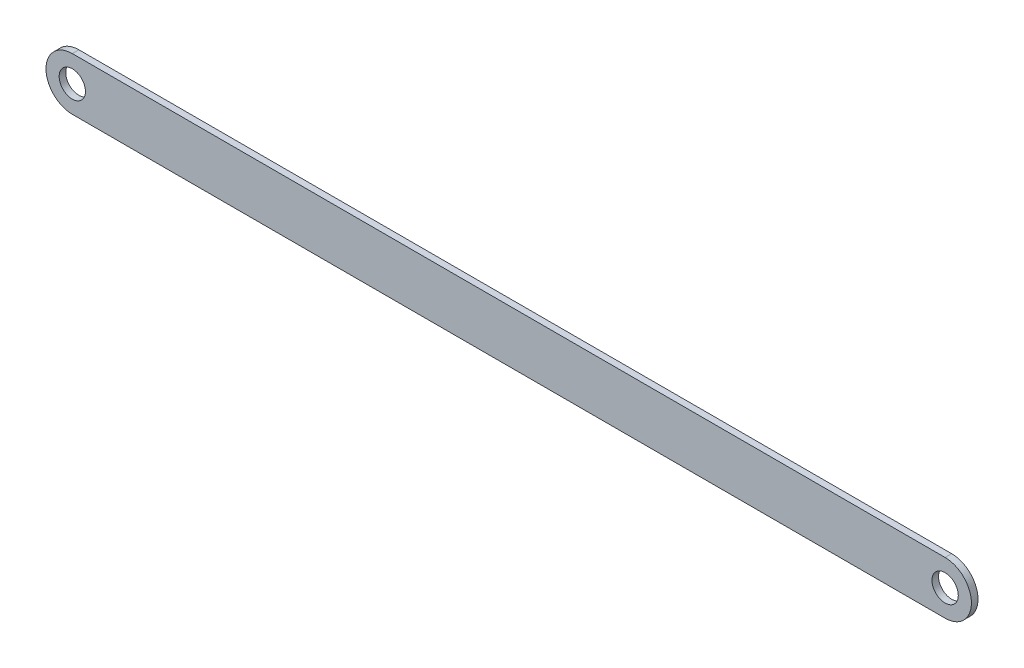
SolidWorks part; units mm, degrees
ref_plane "Front Plane" through (0, 0, 0) normal (0, 0, 1) x (1, 0, 0)
ref_plane "Top Plane" through (0, 0, 0) normal (0, 1, 0) x (1, 0, 0)
ref_plane "Right Plane" through (0, 0, 0) normal (1, 0, 0) x (0, 0, -1)
sketch "Sketch1" plane through (0, 0, 0) normal (0, 0, 1) x (1, 0, 0)
  line L0 (-165.885, 0) -> (165.885, 0) construction
  line L1 (-165.885, 10) -> (165.885, 10)
  line L2 (-165.885, -10) -> (165.885, -10)
  arc A0 (-165.885, 10) -> (-165.885, -10) centre (-165.885, 0) ccw
  arc A1 (165.885, -10) -> (165.885, 10) centre (165.885, 0) ccw
  circle A2 centre (-165.885, 0) radius 5
  circle A3 centre (165.885, 0) radius 5
  point P2 (0, 0)
  dimension "D1" = 331.77
  dimension "D2" = 10
  dimension "D3" = 10
extrude "Boss-Extrude1" add sketch "Sketch1" along normal blind 2.5
